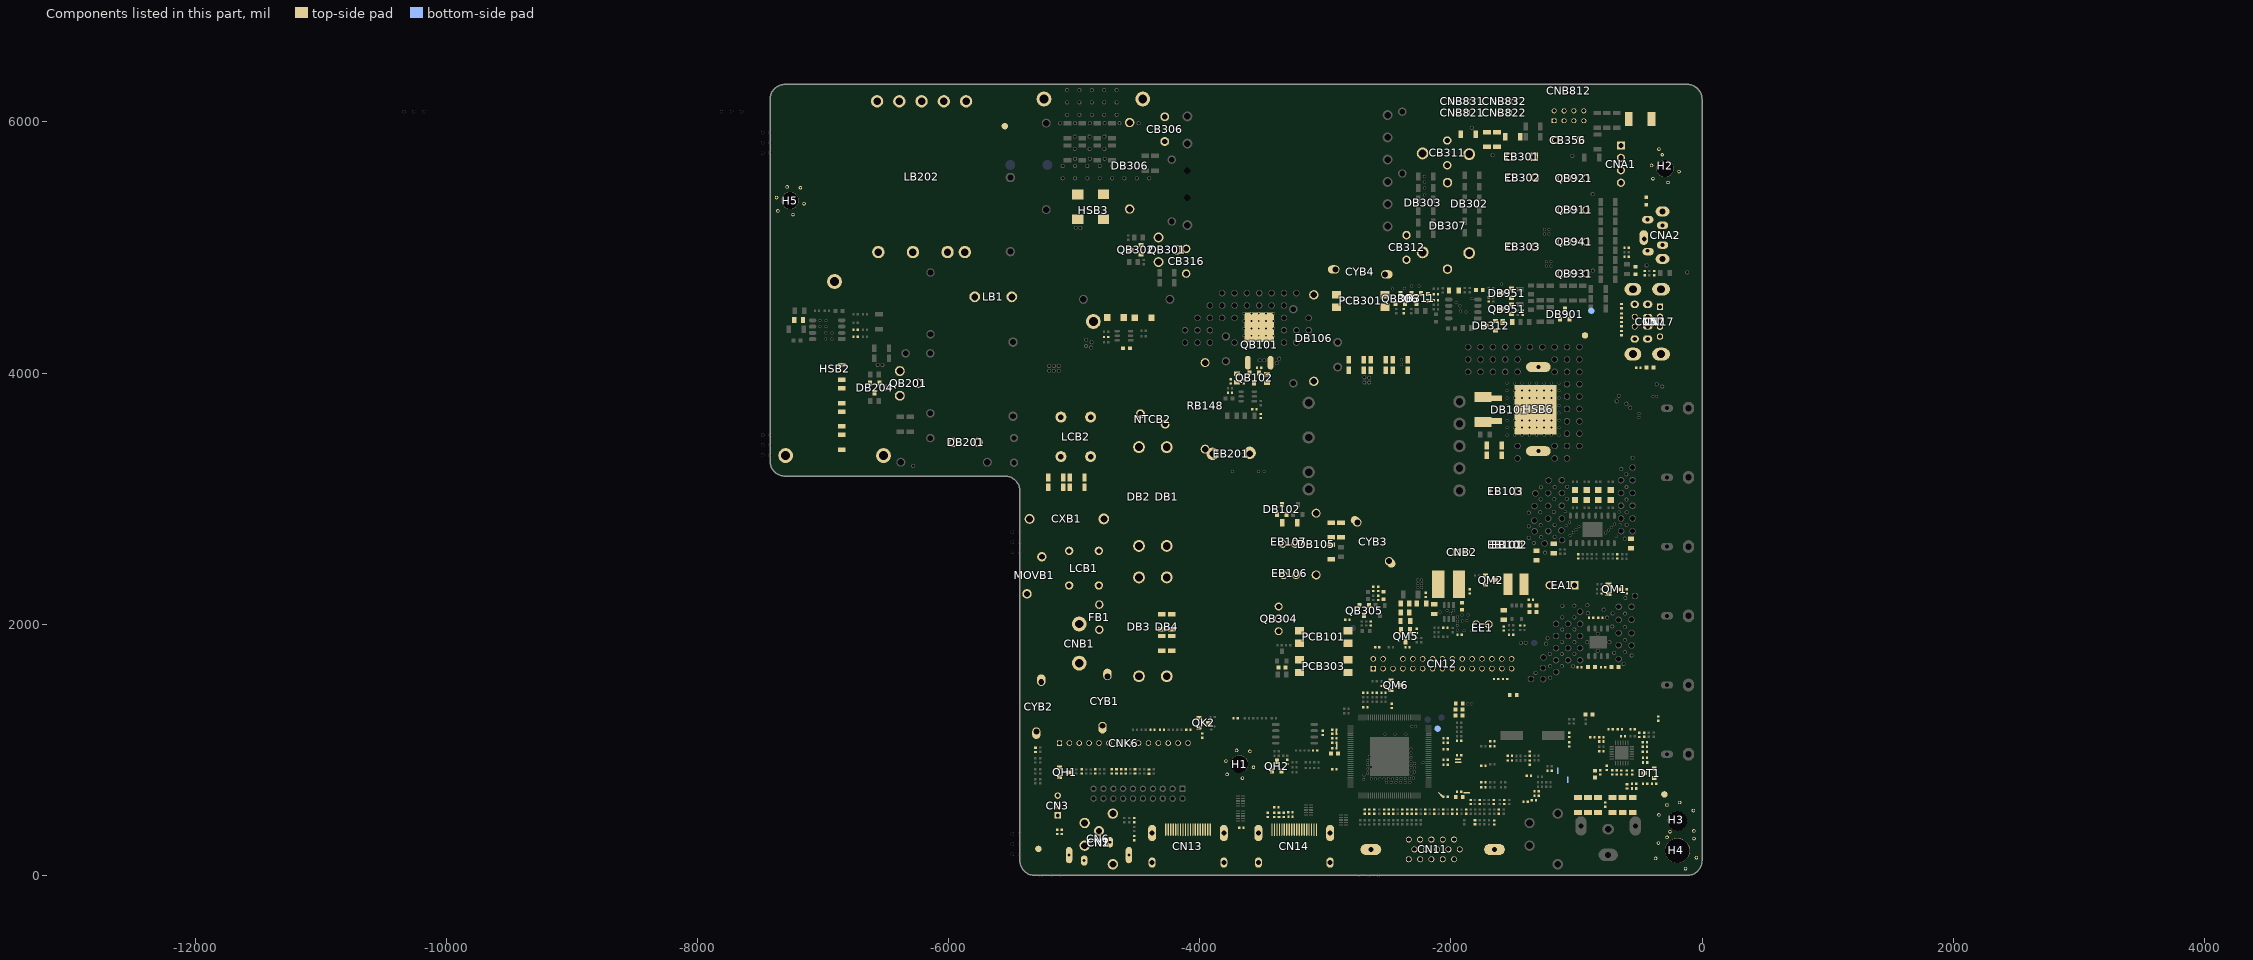
[diagram p0: the components of this part, seen from the top]
# Altium PCB MISC84277.PcbDoc (part 2 of 15)
Units mil, origin at the board's own origin, x right, y up, seen from the top; angles counter-clockwise.
Board outline 7422.08 x 6299.21 mil, 2 copper layers (TopLayer, BottomLayer), stack 61.855 mil thick; 709 components, 395 nets, 2812 pads, 811 vias.

## Components (designator, comment, footprint, x,y, rotation, side; value= is the part's Value field where it differs from the comment) (continued)
CB303 "100pF-0402-NPO-±5%-50V" C0402 -4745.41,4287.55 r180 top
CB304 "0.1uF-0603-X7R-±10%-50V" C0603 -4584.14,4197.94 r0 top
CB305 "100pF-0402-NPO-±5%-50V" C0402 -1699.45,4587.77 r90 top
CB306 "C242G472J20A201 (tape and reel/Faraday)" CAP8*2.5-V-5 -4279.5,5943 r90 top
CB311 "Ceramic capacitor, CAP CD, 1KV, 1000pF, ±10%, Y5R, P, 5.0mm, DIP, TP, SHM" CAP7.5*2.5-V-5 -2030,5754.16 r270 top
CB312 "Ceramic capacitor, CAP CD, 1KV, 100pF, ±10%, SL, P, 5.0mm, DIP, TP, SHM" CAP7.5*2.5-V-5 -2354.06,5000.38 r270 top
CB316 "Ceramic capacitor, CAP CD, 1KV, 100pF, ±10%, SL, P, 5.0mm, DIP, TP, SHM" CAP7.5*2.5-V-5 -4109,4891 r90 top
CB321 "0.1uF-0603-X7R-±10%-50V" C0603 -3346.5,1656.76 r180 top
CB322 "0.022uF-0603-X7R-±10%-25V" C0603 -2184,4602.5 r90 top
CB323 "1000pF-0402-X7R-±10%-50V" C0402 -2120.5,4629.5 r180 top
CB324 "NC/1000pF-0402-X7R-±10%-50V" C0402 -2119.5,4581 r180 top
CB326 "0.33uF-0805-X7R-±10%-50V" C0805 -1977.5,4659 r0 top
CB327 "0.1uF-0402-X7R-±10%-16V" C0402 -2638.95,2005.98 r270 top
CB328 "0.047uF-0805-X7R-±10%-50V" C0805 -1548.5,4407.5 r0 top
CB340 "1000pF-0402-X7R-±10%-50V" C0402 -2375.5,4493.5 r270 top
CB350 "Ceramic capacitor, CAP MC, 25V, 0.47uF, ±10%, X7R, 0603, SMD, TP" C0603 -1774.5,4660.5 r0 top
CB356 "NC/CK45-B3AD102KYPNX(TDK)" CAP8.5*4-V-5 -1069,5856.2 r180 top
CB951 "NC/0.1uF-0402-X7R-±10%-16V" C0402 -1430.12,4480.1 r270 top
CD1 "10uF-0805-X5R-±20%-16V" C0805 -2236.17,2164.33 r180 top
CD2 "1uF-0402-X5R-±20%-6.3V" C0402 -1930.53,1915.44 r180 top
CD3 "0.1uF-0402-X5R-±20%-16V" C0402 -1849.88,2261.42 r90 top
CD4 "10uF-0603-X5R-±20%-6.3V" C0603 -1912.88,2143.31 r90 top
CD5 "10uF-0805-X5R-±20%-16V" C0805 -2132.7,2119.35 r270 top
CD6 "0.1uF-0402-X5R-±20%-16V" C0402 -2202.2,2233.62 r90 top
CD7 "8pF-0402-NPO-±5%-50V" C0402 -2044,1972 r0 top
CD8 "NC/10uF-0805-X5R-±20%-16V" C0805 -1181,2602 r90 top
CD9 "NC/10uF-0805-X5R-±20%-16V" C0805 -565,2643 r270 top
CD10 "10uF-0805-X5R-±20%-16V" C0805 -1318.25,2547.03 r270 top
CD11 "10uF-0805-X5R-±20%-16V" C0805 -1580,2074 r270 top
CD12 "0.1uF-0402-X5R-±20%-16V" C0402 -1580,1966 r270 top
CD13 "NC/NC/3300pF-0402-X7R-±10%-50V" C0402 -1520,1917 r0 top
CD14 "10uF-0603-X5R-±20%-6.3V" C0603 -1347,2149 r0 top
CD15 "10uF-0603-X5R-±20%-6.3V" C0603 -1345,2099 r0 top
CD16 "0.1uF-0402-X5R-±20%-16V" C0402 -1364,2194 r0 top
CD17 "1uF-0402-X5R-±20%-6.3V" C0402 -1431,1990 r0 top
CF1 "30pF-0402-NPO-±5%-50V" C0402 -1670,1069 r180 top
CF2 "0.1uF-0402-X5R-±20%-16V" C0402 -3020,1135 r90 top
CF3 "10uF-0603-X5R-±20%-6.3V" C0603 -2929,970 r180 top
CF4 "30pF-0402-NPO-±5%-50V" C0402 -1670,1028.99 r180 top
CF5 "10uF-0603-X5R-±20%-6.3V" C0603 -1935,1321 r180 top
CF6 "0.1uF-0402-X5R-±20%-16V" C0402 -2471,1350 r270 top
CF7 "0.1uF-0402-X5R-±20%-16V" C0402 -2350,508 r90 top
CF8 "0.1uF-0402-X5R-±20%-16V" C0402 -2929,1091 r0 top
CF9 "0.1uF-0402-X5R-±20%-16V" C0402 -1935,958 r0 top
CF10 "0.1uF-0402-X5R-±20%-16V" C0402 -1935,1071 r180 top
CF11 "0.1uF-0402-X5R-±20%-16V" C0402 -2688,508 r90 top
CF12 "0.1uF-0402-X5R-±20%-16V" C0402 -2041.73,921 r180 top
CF13 "0.1uF-0402-X5R-±20%-16V" C0402 -2041.73,625 r180 top
CF14 "0.1uF-0402-X5R-±20%-16V" C0402 -2041.73,881 r180 top
CF15 "10uF-0603-X5R-±20%-6.3V" C0603 -1934,1369 r180 top
CF16 "1uF-0402-X5R-±20%-6.3V" C0402 -2929,1161 r0 top
CF17 "1uF-0402-X5R-±20%-6.3V" C0402 -2682,1337 r0 top
CF18 "1uF-0402-X5R-±20%-6.3V" C0402 -2929,846 r0 top
CF19 "1uF-0402-X5R-±20%-6.3V" C0402 -2042,1092 r180 top
CF20 "1uF-0402-X5R-±20%-6.3V" C0402 -2041.73,1006 r180 top
CF21 "1uF-0402-X5R-±20%-6.3V" C0402 -2929,1127 r0 top
CF22 "NC/10uF-0603-X5R-±20%-6.3V" C0603 -1935,1273 r180 top
CF23 "1uF-0402-X5R-±20%-6.3V" C0402 -2929,1012 r0 top
CF24 "1uF-0402-X5R-±20%-6.3V" C0402 -2041.73,1056 r180 top
CF25 "1uF-0402-X5R-±20%-6.3V" C0402 -2929,1055 r0 top
CF26 "0.047uF-0402-X7R-±10%-16V" C0402 -1952,507 r270 top
CF27 "0.1uF-0402-X5R-±20%-16V" C0402 -1935,666.8 r180 top
CF28 "10uF-0603-X5R-±20%-6.3V" C0603 -1934,624.8 r0 top
CF29 "NC/1000pF-0402-X7R-±10%-50V" C0402 -1380,793 r180 top
CF30 "NC/1000pF-0402-X7R-±10%-50V" C0402 -1214,834 r180 top
CF31 "0.047uF-0402-X7R-±10%-16V" C0402 -2460,508 r270 top
CF32 "1Kohm-0402-±5%-1/16W" C0402 -1059.06,1118.38 r90 top
CF33 "1000pF-0402-X7R-±10%-50V" C0402 -874.02,1100 r180 top
CF34 "0.047uF-0402-X7R-±10%-16V" C0402 -2205,507 r270 top
CF35 "NC/5pF-0402-NPO-±5%-50V" C0402 -1568.74,1563.82 r180 top
CF36 "NC/5pF-0402-NPO-±5%-50V" C0402 -1639.61,1563.82 r180 top
CF37 "NC/10uF-0603-X5R-±20%-6.3V" C0603 -1504,1436 r0 top
CF38 "NC/NC/30pF-0402-NPO-±5%-50V" C0402 -1059.06,1043.58 r90 top
CF39 "NC/4.7pF-0402-NPO-±5%-50V" C0402 -802,1100 r180 top
CG1 "NC/0.1uF-0402-X5R-±20%-16V" C0402 -2682,1454 r0 top
CG2 "NC/0.1uF-0402-X5R-±20%-16V" C0402 -2608,1454 r0 top
CH3 "NC/0.1uF-0402-X5R-±20%-16V" C0402 -4701.7,828.2 r270 top
CH4 "NC/0.1uF-0402-X5R-±20%-16V" C0402 -4831.7,828.1 r270 top
CH7 "NC/30pF-0402-NPO-±5%-50V" C0402 -3277.9,466.4 r180 top
CH8 "NC/0.1uF-0402-X5R-±20%-16V" C0402 -3458,482 r270 top
CH9 "NC/0.1uF-0402-X5R-±20%-16V" C0402 -3408,482 r90 top
CH10 "NC/30pF-0402-NPO-±5%-50V" C0402 -3669.7,378.1 r180 top
CH15 "NC/1uF-0402-X5R-±20%-6.3V" C0402 -4627.5,828 r270 top
CI1 "0.047uF-0402-X7R-±10%-16V" C0402 -2060,507 r270 top
CI2 "NC/100pF-0402-NPO-±5%-50V" C0402 -1988,507 r90 top
CI3 "1uF-0402-X5R-±20%-6.3V" C0402 -1844,584 r270 top
CI4 "1uF-0402-X5R-±20%-6.3V" C0402 -1772,584 r270 top
CI5 "1uF-0402-X5R-±20%-6.3V" C0402 -1318,669 r0 top
CI6 "1uF-0402-X5R-±20%-6.3V" C0402 -1318,633 r0 top
CI7 "0.047uF-0402-X7R-±10%-16V" C0402 -2278,508 r270 top
CI8 "NC/100pF-0402-NPO-±5%-50V" C0402 -348,1248 r90 top
CI9 "NC/0.047uF-0402-X7R-±10%-16V" C0402 -2314,508 r270 top
CI11 "NC/0.047uF-0402-X7R-±10%-16V" C0402 -2132,507 r270 top
CK1 "NC/0.1uF-0402-X5R-±20%-16V" C0402 -3980.6,1113.2 r90 top
CK2 "0.01uF-0402-X7R-±10%-50V" C0402 -3715,1250.99 r180 top
CK3 "NC/0.1uF-0402-X5R-±20%-16V" C0402 -4091.6,1160.01 r0 top
CK6 "NC/10pF-0402-NPO-±5%-50V" C0402 -4376.9,1160.01 r180 top
CK10 "NC/0.1uF-0402-X5R-±20%-16V" C0402 -4301.2,1160.01 r0 top
CL2 "0.1uF-0402-X5R-±20%-16V" C0402 -884,2052 r0 top
CL3 "0.1uF-0402-X5R-±20%-16V" C0402 -976.38,1657.57 r180 top
CL4 "NC/10uF-0603-X5R-±20%-6.3V" C0603 -881,1659 r0 top
CL42 "0.1uF-0402-X5R-±20%-16V" C0402 -810,2053 r0 top
CL43 "0.1uF-0402-X5R-±20%-16V" C0402 -788.73,1659.01 r0 top
CL44 "10uF-0603-X5R-±20%-6.3V" C0603 -694,1659 r0 top
CM1 "0.22uF-0402-X5R-±10%-16V" C0402 -798,2262 r90 top
CM2 "0.1uF-0402-X5R-±20%-16V" C0402 -601,2262 r270 top
CM3 "NC/0.1uF-0402-X5R-±20%-16V" C0402 -2272,1947 r90 top
CM4 "0.1uF-0402-X5R-±20%-16V" C0402 -2587,1817 r180 top
CM5 "NC/10uF-0805-X5R-±20%-16V" C0805 -2364,2025 r180 top
CM7 "0.022uF-0402-X7R-±10%-16V" C0402 -2346,1816 r0 top
CN1 "RCA terminal, RCA Jack, AV1, H, Yellow, CH5.5, Seal, DIP, AV38A-01S-5030, QS" AV1-H-4 -4803.22,37.25 r0 top locked
CN2 "NC/RCA terminal, RCA Jack, AV1, H, Orange, CH5.5, Seal, DIP, AV38A-01S-5020, QS" AV1-H-4 -4803.22,37.25 r0 top locked
CN3 "NC/3PIN-2.0-D-H-G" SIP3/2.0D-1 -5131.53,556.36 r90 top locked
CN5 "WLUS-074B" USB2-HD-1 78.74,4409.45 r90 top locked
CN6 "NC/earphone terminal, Earphone Jack, H, Φ3.5, CH7.0, Black, switch, Seal, DIP, PJ7724-F05L3BY-D, YUQIU" PHONE-HD-42 -4803.15,-0.15 r0 top locked
CN7 "NC/USB-042M-002DP" USB1-HD-2 76.66,4409.45 r90 top locked
CN11 "WLHD-051A" DB15-HF-1 -2145.67,0.15 r0 top locked
CN12 "2×15PIN-2.0-D-H-M(pin length=2.6mm)-LD(missing 6PIN)" SIP2*15/2.0D-2 -2067.56,1685.43 r180 top
CN13 "161011041" HDMI-HS-1 -4094.49,-78.59 r0 top locked
CN14 "161011041" HDMI-HS-1 -3248.03,-78.59 r0 top locked
CN17 "NC/4PIN-2.0-D-H-G" SIP4/2.0D-1 -335.48,4409 r270 top locked
CNA1 "Connect jack, 4Pin, D2.50, D, L=2.8mm, DIP, LD" SIP4/2.54D-1 -646.5,5664.86 r270 top
CNA2 "PJ-339" PHONE-HD-12 0,5098.43 r90 top locked
CNB1 "Connect jack, 2Pin, D7.92, L, SNAP, Fool-proofing, nature, L=2.8mm, DIP, AMA" CON2-H7.92 -4960.63,1846.02 r0 top
CNB2 "2PIN-2.0-D-H-G-LD" SIP2/2.0D-1 -1913.13,2574.5 r0 top
CNB812 "NC/2×4PIN-2.0-L-H-F-gold plated-LK" SIP2*4H/2.0DF-1 -1060.17,6048.98 r0 top locked
CNB821 "NC/2PIN-2.0-D-H-G-LD" SIP2/2.0D-CP -1911.14,6072.15 r180 top
CNB822 "2PIN-2.0-D-H-G-LD" SIP2/2.0D-CP -1575.87,6072.15 r180 top
CNB831 "NC/3PIN-2.0-D-H-G-LD" SIP3/2.0D-CP -1911.14,6163.14 r180 top
CNB832 "3PIN-2.0-D-H-G-LD" SIP3/2.0D-CP -1575.87,6163.14 r180 top
CNK6 "Connect jack, 14Pin, D2.0, D, L=2.8mm, DIP, LD" SIP14/2.0D-1 -4606,1053.3 r0 top locked
CO1 "NC/1uF-0402-X5R-±20%-6.3V" C0402 -1574,584 r90 top
CO4 "NC/1uF-0402-X5R-±20%-6.3V" C0402 -1618,507 r90 top
CO6 "NC/0.1uF-0402-X5R-±20%-16V" C0402 -5136.7,346.8 r90 top
CO7 "NC/330pF-0402-NPO-±5%-50V" C0402 -5098.6,346.8 r90 top
CO8 "NC/NC/10pF-0402-NPO-±5%-50V" C0402 -3081,994.42 r0 top
CO9 "100pF-0402-NPO-±5%-50V" C0402 -1880,507 r90 top
CO10 "NC/NC/4700pF-0402-X7R-±10%-50V" C0402 -4522.9,439.7 r90 top
CO11 "NC/NC/4700pF-0402-X7R-±10%-50V" C0402 -4522.9,295.9 r90 top
COLD "COLD" COLD -3154.3,628.8 r0 top
CQC "CQC" CQC -555,3635 r270 top
CT1 "0.1uF-0402-X5R-±20%-16V" C0402 -802.12,989.41 r0 top
CT2 "NC/10uF-0603-X5R-±20%-6.3V" C0603 -899,1281.8 r0 top
CT5 "0.1uF-0402-X5R-±20%-16V" C0402 -809.75,820.98 r90 top
CT6 "10uF-0603-X5R-±20%-6.3V" C0603 -851.63,805.39 r270 top
CT7 "30pF-0402-NPO-±5%-50V" C0402 -460.97,1119.86 r270 top
CT8 "30pF-0402-NPO-±5%-50V" C0402 -455.62,1058.41 r180 top
CT9 "0.1uF-0402-X5R-±20%-16V" C0402 -557.5,819.42 r270 top
CT10 "33pF-0402-NPO-±5%-50V" C0402 -1371.94,969.79 r90 top
CT11 "0.022uF-0402-X7R-±10%-16V" C0402 -679.97,820.36 r90 top
CT12 "0.022uF-0402-X7R-±10%-16V" C0402 -715.97,820.36 r270 top
CT13 "NC/1.2pF-0402-NPO-±0.25pf-50V" C0402 -540.73,730.27 r0 top
CT17 "NC/100pF-0402-NPO-±5%-50V" C0402 -454.08,730.26 r180 top
CT18 "0.1uF-0402-X5R-±20%-16V" C0402 -759.1,855.98 r90 top
CT19 "NC/0.022uF-0402-X7R-±10%-16V" C0402 -1742,874 r0 top
CT20 "0.1uF-0402-X5R-±20%-16V" C0402 -1531,951.29 r180 top
CT21 "0.047uF-0402-X7R-±10%-16V" C0402 -455.62,1022.41 r0 top
CT23 "0.1uF-0402-X5R-±20%-16V" C0402 -1531,914.79 r180 top
CT24 "33pF-0402-NPO-±5%-50V" C0402 -1372,898 r90 top
CT25 "0.1uF-0402-X5R-±20%-16V" C0402 -498.92,1118.68 r90 top
CT26 "330pF-0402-NPO-±5%-50V" C0402 -629.92,1107.68 r0 top
CT27 "0.1uF-0402-X5R-±20%-16V" C0402 -655.4,1162.47 r0 top
CT29 "6800pF-0402-X7R-±10%-50V" C0402 -552.9,1162.49 r0 top
CT30 "0.1uF-0402-X5R-±20%-16V" C0402 -729,1163 r0 top
CT40 "470pF-0402-X7R-±10%-50V" C0402 -770.21,563.26 r90 top
CT41 "0ohm-1206-±5%-1/4W" C1206 -828.71,559.76 r270 top
CT42 "0ohm-1206-±5%-1/4W" C1206 -632.21,560.76 r270 top
CT43 "0ohm-1206-±5%-1/4W" C1206 -712.21,560.76 r270 top
CT44 "0ohm-1206-±5%-1/4W" C1206 -908.71,559.76 r270 top (schematic designator CT43)
CT45 "NC/4700pF-1206-X7R-±10%-1000V" C1206 -988.71,559.76 r270 top
CT46 "NC/4700pF-1206-X7R-±10%-1000V" C1206 -552.21,560.76 r270 top
CU1 "10uF-0603-X5R-±20%-6.3V" C0603 -414,4045.5 r180 top
CV1 "0.047uF-0402-X7R-±10%-16V" C0402 -2387,508 r270 top
CV3 "0.047uF-0402-X7R-±10%-16V" C0402 -2496,508 r270 top
CV5 "1uF-0402-X5R-±20%-6.3V" C0402 -1742,701 r180 top
CV6 "1uF-0402-X5R-±20%-6.3V" C0402 -1742,739.99 r180 top
CV7 "0.047uF-0402-X7R-±10%-16V" C0402 -2532,508 r270 top
CV9 "33pF-0402-NPO-±5%-50V" C0402 -2610,508 r270 top
CV10 "33pF-0402-NPO-±5%-50V" C0402 -2649,508 r270 top
CXB1 "X capacitor, CAP X2, MP, 275VAC, 0.47uF, ±10%, S, 15mm-Mini, PC, DIP, BM" CAP18*8.5-V-15 -5060.1,2838.9 r180 top
CYB1 "CD70-B2GA221KYPKA(S/TDK)" CAP13*4.5-V-10 -4755.5,1388.55 r90 top
CYB2 "CD70-B2GA221KYPKA(S/TDK)" CAP13*4.5-V-10 -5282.5,1343.5 r90 top
CYB3 "CD85-B2GA471KYPKA(S/TDK)" CAP13*4.5-V-10 -2619.94,2655.96 r315 top
CYB4 "CD85-B2GA471KYPKA(S/TDK)" CAP13*4.5-V-10 -2722,4806 r0 top
DB1 "1N5408G (tape and reel / GOOD-ARK)" D3-H-20 -4263.49,3016.92 r90 top locked
DB2 "1N5408G (tape and reel / GOOD-ARK)" D3-H-20 -4484.49,3016.92 r90 top locked
DB3 "1N5408G (tape and reel / GOOD-ARK)" D3-H-20 -4484.49,1979.42 r90 top
DB4 "1N5408G (tape and reel / GOOD-ARK)" D3-H-20 -4263.49,1979.42 r90 top
DB101 "MBRB10150CT(GOOD-ARK)" D2PAK3 -1328.33,3709.25 r270 top
DB102 "LBAV70LT1G(LRC)" SO-23 -3347,2915.5 r180 top
DB105 "FR107 (tape and reel/LRC)" D1-H-12.5 -3074,2638.5 r270 top
DB106 "FR207 (tape and reel/LRC)" D2-H-17.5 -3092,4278.68 r270 top
DB201 "Rectifier diode, DIO FRD S, 8A, 600V, ITO-220AC, DIP, UGF8J C0G, TSC" TO-220-AK-H -5865.59,4118.29 r0 top locked
DB202 "NC/GS3J-B(GULF)" DIODE-SMB-1 -4971.94,5323.42 r270 top
DB203 "NC/GS3J-B(GULF)" DIODE-SMB-1 -4766.44,5323.92 r270 top
DB204 "LBAV70LT1G(LRC)" SO-23 -6589.92,3881.88 r0 top
DB302 "Rectifier diode, DIO FRD S, 4A, 800V, DO-201AD, DIP, MUR480-84mil, GOOD-ARK" D3-H-20 -1854.4,5350.09 r270 top
DB303 "Rectifier diode, DIO FRD S, 4A, 800V, DO-201AD, DIP, MUR480-84mil, GOOD-ARK" D3-H-20 -2225.5,5355.39 r270 top locked
DB306 "FR207 (tape and reel/LRC)" D2-H-17.5 -4559,5651 r90 top
DB307 "FR207 (tape and reel/LRC)" D2-H-17.5 -2027.5,5172.66 r90 top
DB310 "M7(WEJ)" DIODE-S-2 -493.55,6024.8 r180 top
DB311 "LBAV70LT1G(LRC)" SO-23 -2275,4594.5 r0 top
DB312 "BAW56(NXP)" SO-23-1 -1685.5,4377 r90 top
DB370 "NC/FF7" DIODE-S-14 -4670.25,4443.16 r180 top
DB371 "NC/FF7" DIODE-S-14 -4450.79,4442 r180 top
DB901 "NC/LBAV70LT1G(LRC)" SO-23 -1093.5,4469 r180 top
DB951 "NC/LBAV70LT1G(LRC)" SO-23 -1557.68,4636.79 r270 top
DDR_1V8 "TEST" TP -2106,1168 r180 bottom
DH1 "NC/NC/AVLC18S02003" DIODE-S0402 -3304.6,903.2 r270 top
DH2 "NC/NC/AVLC18S02003" DIODE-S0402 -3389.9,541.4 r0 top
DH3 "NC/NC/AVLC18S02003" DIODE-S0402 -4590.4,827.6 r90 top
DH4 "NC/NC/AVLC18S02003" DIODE-S0402 -4404.7,826.1 r90 top
DH5 "NC/NC/AVLC18S02003" DIODE-S0402 -4516.6,828.5 r90 top
DH6 "NC/NC/AVLC18S02003" DIODE-S0402 -3332,482 r90 top
DH7 "NC/NC/AVLC18S02003" DIODE-S0402 -3370,482 r90 top
DH8 "NC/NC/AVLC18S02003" DIODE-S0402 -4664.5,827.8 r270 top
DH9 "NC/NC/AVLC18S02003" DIODE-S0402 -4940.9,827.5 r270 top
DH10 "NC/NC/AVLC18S02003" DIODE-S0402 -3278.23,503.7 r180 top
DK1 "NC/AVLC18S02003" DIODE-S0402 -5308.96,999.63 r90 top
DT1 "BAV99-BR" SO-23 -421.12,814.41 r270 top
DU1 "NC/AIES12U020R2" DIODE-S0402 -1808,423 r270 top (schematic designator DH7)
DU3 "NC/AIES12U020R2" DIODE-S0402 -641.5,4458 r90 top
DU4 "NC/AIES12U020R2" DIODE-S0402 -641.5,4532.5 r270 top
DU7 "NC/AIES12U020R2" DIODE-S0402 -641.5,4318.5 r90 top
DU8 "NC/AIES12U020R2" DIODE-S0402 -641.5,4389.5 r270 top
EA1 "470uF-16V±20%-10×12-105℃-tape and reel-F=5.0-XL" EC(10*12)-V-5 -1114.5,2311.16 r180 top
EB101 "470uF-25V-±20%-10×12.5-105℃-GF-tape and reel-F=5.0 (CapXon)" EC(10*12.5)-V-5 -1563.34,2633.4 r180 top
EB102 "NC/270uF-16V-±20%-8×11.5-105℃-PS-short leads-F=3.5 (Capxon)" EC(8*11)-V-3.5 -1533.82,2633.4 r180 top
EB103 "470uF-25V-±20%-10×12.5-105℃-GF-tape and reel-F=5.0 (CapXon)" EC(10*12.5)-V-5 -1564.32,3058.4 r180 top locked
EB106 "47uF-50V-±20%-6.3×11-105℃-GH-tape and reel-F=2.5 (CapXon)" EC(6.3*11)-V-2.5#1 -3283.25,2390.43 r180 top
EB107 "10uF-50V-±20%-5×11-105℃-GH-tape and reel-F=2.5 (CapXon)" EC(5*11)-V-2.5 -3290.87,2640.07 r180 top
EB201 "100uF-450V-±20%-16×35.5-105℃-KM-bent leads (H=8.1mm) (Capxon)" EC(16*37)-H-7.5 -3750.19,3357 r0 top locked
EB301 "33uF-250V-±20%-13×20-105℃-FK-tape and reel-F=5.0 (Capxon)" EC(13*20)-H-5 -1437.15,5721.67 r0 top locked
EB302 "NC/aluminum electrolytic capacitor, CAP AL, 200V, 33uF, ±20%, LD, KF, P, 5.0mm, 13×13, DIP, TP, CapXon" EC(13*13)-V-5 -1430.05,5557.67 r180 top locked
EB303 "NC/aluminum electrolytic capacitor, CAP AL, 200V, 33uF, ±20%, LD, KF, P, 5.0mm, 13×13, DIP, TP, CapXon" EC(13*13)-V-5 -1430.05,5005.3 r180 top locked
EE1 "470uF-10V-±20%-6.3×11-105℃-black base white print-tape and reel-F=2.5-XF" EC(6.3*11)-V-2.5#2 -1749.49,1999.61 r180 top locked
EVA1 "NC/7×7×3mm-C-4305 fireproof foam-black" EVA(7*7*3) -1747.5,5341.3 r180 bottom
EVA2 "NC/7×7×3mm-C-4305 fireproof foam-black" EVA(7*7*3) -6971.04,3455.13 r180 bottom
EVA3 "NC/7×7×3mm-C-4305 fireproof foam-black" EVA(7*7*3) -6548.87,5829.14 r180 bottom
EVA4 "NC/7×7×3mm-C-4305 fireproof foam-black" EVA(7*7*3) -2176.6,3326.3 r180 bottom
EVA5 "NC/7×7×3mm-C-4305 fireproof foam-black" EVA(7*7*3) -5239,848.6 r180 bottom
EVA6 "NC/7×7×3mm-C-4305 fireproof foam-black" EVA(7*7*3) -1388.05,984.65 r180 bottom
EVA7 "NC/7×7×3mm-C-4305 fireproof foam-black" EVA(7*7*3) -548.56,2006.31 r180 bottom
F2 "0ohm-0402-±5%-1/16W" R0402 -508,4044 r0 top
FB1 "2010T3.15A250VA1 (tape and reel/Huade)" FUSE8.5*4-V-5 -4800.5,2056.41 r270 top
GD1 "7.00×8.35mm-nylon-white-WQM" Fixed -7204.72,6082.68 r0 top locked
GD2 "7.00×8.35mm-nylon-white-WQM" Fixed -5000,1279.53 r0 top locked
GD3 "7.00×8.35mm-nylon-white-WQM" Fixed -2814.96,2303.15 r0 top locked
GD4 "7.00×8.35mm-nylon-white-WQM" Fixed -2185.04,5964.57 r0 top locked
GL1 "SLD-8854W" "Silica gel-20" -4085.1,2485.6 r0 top
GL2 "SLD-8854W" "Silica gel-10" -1436.65,5249.36 r180 top
GL3 "NC/SLD-8854W" "Silica gel-10" -5872.05,4415.35 r45 top
GL4 "SLD-8854W" "Silica gel-10" -5862.2,3862.2 r0 top
H1 "Location hole" ASSE3.5C-3#1 -3685.04,885.98 r0 top locked
H2 "Location hole" ASSE3.5C-3#2 -295.28,5629.92 r0 top locked
H3 "Location hole" ASSE4.0C-4 -196.85,433.22 r0 top locked
H4 "Location hole" ASSE5.0C-4 -196.85,197 r0 top locked
H5 "Location hole" ASSE3.5C-3#1 -7264.15,5374.17 r0 top locked (schematic designator H6)
"High Voltage" "High Voltage" "High Voltage" -4779.9,1821.1 r0 top
HOT "HOT" HOT -4852.28,3957.09 r0 top
HS "NC/14×14×06-THD" HS-S -2357,1382 r0 top
HSB2 "40×25×5.0-black-with pins (thickness=1.5mm)-FR" HS018 -6909,4036 r0 top locked
HSB3 "50×25×5.0-black-with pins (thickness=1.5mm)-FR" HS033 -4847.99,5297.33 r0 top locked
HSB6 "NC/17.5×14.5×0.5- natural finish -Cu-MRD" HS038 -1304,3713 r90 top
JB102 "NC/0ohm-1206-±5%-1/4W" R1206 -1861.6,5901.27 r0 top
JB103 "NC/0ohm-1206-±5%-1/4W" R1206 -1713.1,5860.2 r90 top
JB106 "NC/0ohm-1206-±5%-1/4W" R1206 -1632.9,5860.6 r90 top
JB107 "NC/0ohm-1206-±5%-1/4W" R1206 -1506.97,5881.7 r180 top
LB1 "SYDR1212-L003-EDL" L/LC2/15*14.5-V7.5 -5645,4607.5 r180 top
LB202 "SYEQ2612-L250uA-SQ" T/EQ2512*11 -6216,5458 r90 top locked
LBA1 "UPZ2012E601-2R0TF(600ohm-2000mA)" L0805 -1012,3028 r90 top
LBA2 "UPZ2012E601-2R0TF(600ohm-2000mA)" L0805 -920,3028 r90 top
LBA3 "UPZ2012E601-2R0TF(600ohm-2000mA)" L0805 -827,3028 r90 top
LBA4 "UPZ2012E601-2R0TF(600ohm-2000mA)" L0805 -728,3028 r90 top
LCB1 "SYT10-L002-EDL" L/LC4/13.5*10-V-7*6 -4922.6,2446.5 r0 top
LCB2 "SYT14-L003-JM" L/LC4/T14-H-8*6 -4988,3492.54 r0 top locked
LD2 "SCD43TL-6R8M" L(4.5*3.5)-S -1482,2319 r0 top
LD12 "Power inductor, Power Inductor, 4.7uH, ±20%, 2.8A, 0.35×1P, DR5.8×4.5, SMD, CD54-4.7uH, wenshan" L(5.8*4.5)-S -2018.7,2318.35 r180 top
LF1 "NC" GND -1943.8,926.4 r0 top
LF2 "NC" GND -2082.8,642.7 r135 top
LF3 "NC" GND -1942.7,902.1 r0 top
LF4 "NC" GND -2912.74,1144.31 r90 top
LF5 "NC" GND -2910.9,1035.2 r270 top
LF6 "NC" GND -1875.4,658.4 r0 top
LF7 "0ohm-0402-±5%-1/16W" L0402 -802,1065.26 r0 top
LT1 "SDCL1005C68NJTDF(68nH-0402±5%-C)" L0402 -600.14,819.42 r90 top
LT2 "GZ1005U102CTF(1000ohm-300mA)" L0402 -642.74,819.42 r270 top
LT3 "0ohm-0402-±5%-1/16W" L0402 -540.74,692.26 r0 top
LT6 "GZ1005U102CTF(1000ohm-300mA)" L0402 -454.09,899.46 r0 top
LT8 "GZ1005U102CTF(1000ohm-300mA)" L0402 -454.71,937.39 r0 top
LT9 "NC/SDCL1005CR27JTDF (Sunlord)" L0402 -382,730.27 r180 top
LT10 "SDCL1005CR18JTDF(180nH-0402±5%-C)" L0402 -455.47,985.36 r0 top
LT11 "NC/SDCL1005CR27JTDF (Sunlord)" L0402 -598,708.64 r90 top
M1 "MARK" MARK -300,645 r0 top
M2 "MARK" MARK -5553.15,5966.54 r0 top
M3 "MARK" MARK -5285.6,211 r0 top
M4 "MARK" MARK -932.6,4300.1 r0 top
Manufacture_Info "Manufacture_Info" MANUFACTURE_INFO -1448.91,3748.36 r0 top
MB1 "PM3.0×8.0×5.5mm-silver-double washer" SCREW -2875.88,5779.23 r0 top
MB2 "PM3.0×8.0×5.5mm-silver-double washer" SCREW -2875.88,5779.23 r0 top
ML1 "Mylar sheet, Mylar, XXX" Mylar -2877.85,5763.97 r90 top
MOVB1 "TVR10561KSC3AGGW (short leads/Weiqin)" VR(13*5)-V-7.5 -5317.6,2389.6 r270 top
"NO DOLBY" "NO DOLBY" "NO DOLBY-SILK" -3460.92,941.68 r0 bottom
NTCB2 "SCK102R55AMBY502 (short leads/Weiqin)" NTC(10*5)-V5 -4374.5,3634 r0 top
PCB101 "LTV-817S-TA-B (Lite-On)" OC4-S-1 -3013,1899.5 r90 top
PCB301 "LTV-817S-TA-B (Lite-On)" OC4-S-1 -2718,4574.5 r90 top
PCB303 "LTV-817S-TA-B (Lite-On)" OC4-S-1 -3013,1665.5 r90 top
PWM_REF "TEST" TP_BL -881.89,4496.06 r0 bottom
QB101 "MOSFET, NMOS, 5A, 700V, 0.9ohm@ID=2.5A@VGS=10V, TO-252, MMD70R900PRH, MAGNACHIP" TO-252-GDS -3527.55,4366.46 r0 top
QB102 "3CG3906M" SOT-23 -3566.5,3960.5 r0 top
QB201 "MDF13N50BTH(Magnachip)" TO-220-GDS-H -7038.92,3917.89 r90 top
QB201和散热片之间 "0.05g" PCB_TIME -2877.85,5763.97 r90 top
QB301 "MDF7N65BTH(Magnachip)" TO-220-GDS-H -4977.91,4982.37 r90 top locked
QB301和散热片之间 "0.05g" PCB_TIME -2877.85,5763.97 r90 top
QB302 "3CG3906M" SOT-23 -4510,4981.5 r270 top
QB304 "2N4401 (Bluearrow)" TO-92-EBC -3372.5,2043 r270 top
QB305 "LMBT3904LT1G" SOT-23 -2690.94,2108.27 r0 top
QB306 "3CG3906M" SOT-23 -2403.5,4594.5 r180 top
QB911 "NC/2SD1857L-Q-T9N-B(UTC)" TO-92-ECB -1022.5,5299.38 r0 top
QB921 "NC/2SD1857L-Q-T9N-B(UTC)" TO-92-ECB -1022.5,5552.73 r0 top
QB931 "NC/2SD1857L-Q-T9N-B(UTC)" TO-92-ECB -1022.5,4792.7 r0 top
QB941 "NC/2SD1857L-Q-T9N-B(UTC)" TO-92-ECB -1022.5,5046.04 r0 top
QB951 "NC/LMBT3904LT1G" SOT-23 -1557.68,4508.88 r270 top
QH1 "LMBT3904LT1G" SOT-23 -5076.3,820.08 r90 top
QH2 "LMBT3904LT1G" SOT-23 -3387.7,870.9 r180 top
QK2 "LMBT3904LT1G" SOT-23 -3967.4,1214.3 r90 top
QM1 "WPM2341A-3/TR" SOT-23-1 -699,2278 r90 top
QM2 "LMBT3904LT1G" SOT-23 -1684,2352 r90 top
QM5 "ME2325-G" SOT-23-1 -2362,1905 r0 top
QM6 "LMBT3904LT1G" SOT-23 -2438,1515 r90 top
R1 "NC/0ohm-0402-±5%-1/16W" R0402 -1340,597 r180 top
R2 "NC/0ohm-0402-±5%-1/16W" R0402 -1406,587 r180 top
R3 "0ohm-0402-±5%-1/16W" R0402 -1655,421.27 r90 top
R4 "0ohm-0402-±5%-1/16W" R0402 -1661,584 r90 top
R5V "NC/0ohm-0805-±5%-1/8W" R0805 -2365,2093 r180 top
R12V "0ohm-0805-±5%-1/8W" R0805 -2364.7,2164.35 r180 top
RA1 "4K7ohm-0402-±5%-1/16W" R0402 -2537,1454 r0 top
RA4 "1Kohm-0402-±5%-1/16W" R0402 -986,2540.5 r90 top
RA7 "NC" GND -1148,831.45 r270 bottom
RA8 "4K7ohm-0402-±5%-1/16W" R0402 -2537,1508 r180 top
RA9 "NC/120ohm-0402-±5%-1/16W" R0402 -456.29,4796.49 r90 top
RA10 "NC/0ohm-0603-±5%-1/10W" R0603 -531.6,4817.8 r90 top
RA11 "NC" GND -1069,762 r270 bottom
RA12 "1Kohm-0402-±5%-1/16W" R0402 -675,2540.5 r90 top
RA14 "NC/120ohm-0402-±5%-1/16W" R0402 -600.22,4997.8 r0 top
RA17 "NC/0ohm-0603-±5%-1/10W" R0603 -444.88,5370.08 r90 top
RA23 "1Kohm-0402-±5%-1/16W" R0402 -382.79,4796.49 r270 top
RA28 "1Kohm-0402-±5%-1/16W" R0402 -600.22,4924.87 r180 top
RB1 "1M2ohm-1206-±5%-1/4W" R1206 -4977.69,3169.17 r180 top
RB2 "1M2ohm-1206-±5%-1/4W" R1206 -4977.69,3090.94 r180 top
RB3 "1M2ohm-1206-±5%-1/4W" R1206 -5148.39,3169.17 r180 top
RB4 "1M2ohm-1206-±5%-1/4W" R1206 -5148.39,3090.94 r180 top
RB101 "330Kohm-1206-±5%-1/4W" R1206 -4304.29,2019.7 r270 top
RB102 "330Kohm-1206-±5%-1/4W" R1206 -4304.29,1847.41 r270 top
RB103 "10Kohm-0402-±1%-1/16W" R0402 -3759.5,3843 r0 top
RB104 "47Kohm-0402-±1%-1/16W" R0402 -3565,3713.5 r0 top
RB105 "510ohm-0402-±5%-1/16W" R0402 -3755,3933.5 r90 top
RB106 "68ohm-0805-±5%-1/8W" R0805 -3702.9,3959.76 r90 top
RB107 "510ohm-0402-±5%-1/16W" R0402 -3650.9,3933.76 r90 top
RB108 "20ohm-0805-±5%-1/8W" R0805 -3464.9,3956.76 r90 top
RB109 "10Kohm-0402-±5%-1/16W" R0402 -3527.55,4042.75 r0 top
RB110 "10ohm-1206-±5%-1/4W" R1206 -3283,2807.5 r0 top
RB114 "10ohm-1206-±5%-1/4W" R1206 -2954.5,2750.5 r90 top
RB115 "10ohm-1206-±5%-1/4W" R1206 -2875.97,2750.5 r90 top
RB116 "10ohm-1206-±5%-1/4W" R1206 -2954.39,2575.32 r270 top
RB117 "10ohm-1206-±5%-1/4W" R1206 -2754.4,4105.75 r180 top
RB118 "10ohm-1206-±5%-1/4W" R1206 -2754.4,4022 r180 top
RB123 "47ohm-1206-±5%-1/4W" R1206 -1654.54,3344.78 r0 top
RB124 "47ohm-1206-±5%-1/4W" R1206 -1654.54,3423.52 r0 top
RB131 "2Kohm-0603-±5%-1/10W" R0603 -2537.4,2230.31 r90 top
RB132 "3Kohm-0402-±1%-1/16W" R0402 -2824.8,2037.4 r180 top
RB133 "3Kohm-0402-±1%-1/16W" R0402 -2618.11,2281.5 r270 top
RB134 "4K7ohm-0402-±1%-1/16W" R0402 -2580.71,2281.5 r90 top
RB135 "18Kohm-0402-±1%-1/16W" R0402 -2580.71,2210.63 r90 top
RB141 "NC/2Mohm-1206-±5%-1/4W" R1206 -4224.49,2019.7 r90 top
RB142 "NC/2Mohm-1206-±5%-1/4W" R1206 -4224.49,1847.41 r90 top
RB143 "NC/0ohm-0402-±5%-1/16W" R0402 -3513,3658.5 r90 top
RB144 "100Kohm-1206-±5%-1/4W" R1206 -2579.32,4105.75 r0 top
RB145 "100Kohm-1206-±5%-1/4W" R1206 -2404.25,4105.75 r0 top
RB146 "100Kohm-1206-±5%-1/4W" R1206 -2579.33,4022 r0 top
RB147 "100Kohm-1206-±5%-1/4W" R1206 -2404.25,4022 r0 top
RB148 "MOF-0R27ohm-±5%-2WS (tape and reel/Futaba)" R2-H-17.5 -3958.38,3739.16 r90 top
RB201 "1Mohm-1206-±1%-1/4W" R1206 -6853,3448.76 r90 top
RB202 "1Mohm-1206-±1%-1/4W" R1206 -6853,3634.34 r90 top
RB203 "1Mohm-1206-±1%-1/4W" R1206 -6853,3819.92 r90 top
RB204 "1Mohm-1206-±1%-1/4W" R1206 -6853,4005.5 r90 top
RB205 "560kohm-0402-±1%-1/16W" R0402 -6741.19,4290 r0 top
RB206 "27Kohm-0402-±1%-1/16W" R0402 -6741.19,4345.31 r180 top
RB209 "39Kohm-0805-±1%-1/8W" R0805 -7194.63,4421.55 r180 top